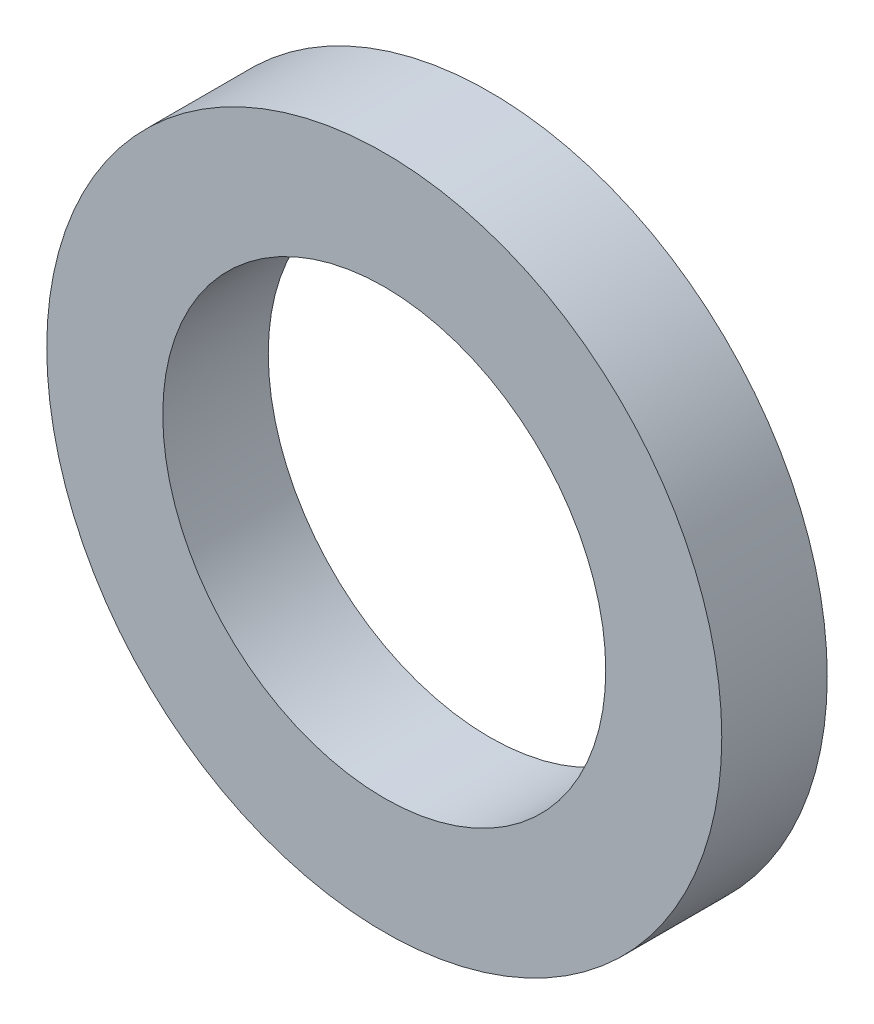
SolidWorks part; units mm, degrees
ref_plane "Front Plane" through (0, 0, 0) normal (0, 0, 1) x (1, 0, 0)
ref_plane "Top Plane" through (0, 0, 0) normal (0, 1, 0) x (1, 0, 0)
ref_plane "Right Plane" through (0, 0, 0) normal (1, 0, 0) x (0, 0, -1)
sketch "Sketch1" plane through (0, 0, 0) normal (0, 0, 1) x (1, 0, 0)
  circle A0 centre (0, 0) radius 1.05
  circle A1 centre (0, 0) radius 1.6
  dimension "D1" = 2.1
  dimension "D2" = 3.2
extrude "Boss-Extrude1" add sketch "Sketch1" along normal mid plane 0.5
